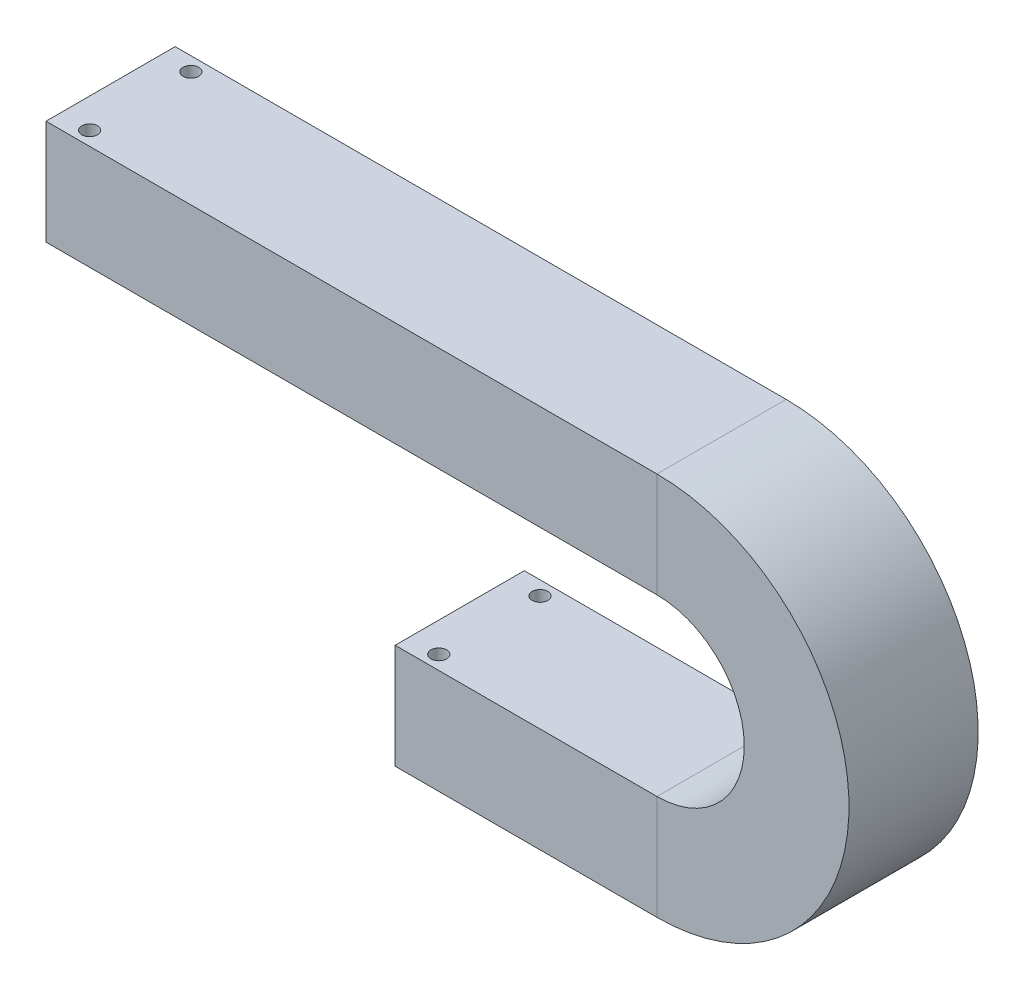
SolidWorks part; units mm, degrees
material "6061-T6"
ref_plane "Front Plane" through (0, 0, 0) normal (0, 0, 1) x (1, 0, 0)
ref_plane "Top Plane" through (0, 0, 0) normal (0, 1, 0) x (1, 0, 0)
ref_plane "Right Plane" through (0, 0, 0) normal (1, 0, 0) x (0, 0, -1)
sketch "Sketch1" plane through (0, 0, 0) normal (1, 0, 0) x (0, 0, -1)
  line L1 (-10, -10) -> (10, -10)
  line L2 (-10, -10) -> (-10, 10)
  line L3 (-10, 10) -> (10, 10)
  line L4 (10, -10) -> (10, 10)
  line L5 (-10, -10) -> (10, 10) construction
  line L6 (-10, 10) -> (10, -10) construction
  line L7 (-18.5, -15) -> (18.5, -15)
  line L8 (-18.5, -15) -> (-18.5, 15)
  line L9 (-18.5, 15) -> (18.5, 15)
  line L10 (18.5, -15) -> (18.5, 15)
  line L11 (-18.5, -15) -> (18.5, 15) construction
  line L12 (-18.5, 15) -> (18.5, -15) construction
  point P0 (0, 0)
  point P6 (0, 0)
  dimension "D1" = 20
  dimension "D2" = 20
  dimension "D3" = 30
  dimension "D4" = 37
sketch "Sketch2" plane through (0, 0, 0) normal (0, 0, 1) x (1, 0, 0)
  line L0 (0, 0) -> (75, 0)
  line L1 (75, 80) -> (-100, 80)
  arc A0 (75, 0) -> (75, 80) centre (75, 40) ccw
  dimension "D1" = 80
  dimension "D2" = 75
  dimension "D3" = 175
sweep "Sweep1" add profiles "Sketch1" path "Sketch2"
hole_wizard "M4 Clearance Hole1" positions "Sketch3" profile "Sketch4" hole size "M4" standard "GB"
sketch "Sketch3" plane through (0, 15, 0) normal (0, 1, 0) x (1, 0, 0)
  line L0 (0, 0) -> (130, 0) construction
  line L1 (130, -18.5) -> (130, 18.5) construction
  line L3 (0, 18.5) -> (0, -18.5) construction
  point P0 (8.5, 14.5)
  point P2 (8.5, -14.5)
  dimension "D1" = 29
  dimension "D2" = 8.5
sketch "Sketch4" plane through (8.5, 15, -14.5) normal (1, 0, 0) x (0, 0, 1)
  line L0 (0, 0) -> (0, 30)
  line L1 (0, 30) -> (2.25, 30)
  line L2 (2.25, 30) -> (2.25, 0)
  line L5 (2.25, 0) -> (0, 0)
  line L11 (0, -6.35) -> (0, 107.95) construction
  dimension "通孔孔直径" = 4.5
  dimension "通孔孔深度" = 30
hole_wizard "M4 Clearance Hole2" positions "Sketch5" profile "Sketch6" hole size "M4" standard "GB" end condition through all
sketch "Sketch5" plane through (0, 95, 0) normal (0, 1, 0) x (1, 0, 0)
  line L0 (-100, 0) -> (130, 0) construction
  line L1 (-100, -18.5) -> (-100, 18.5) construction
  line L2 (130, -18.5) -> (130, 18.5) construction
  point P8 (-91.5, 14.5)
  point P10 (-91.5, -14.5)
  dimension "D1" = 29
  dimension "D2" = 8.5
sketch "Sketch6" plane through (-91.5, 95, 14.5) normal (1, 0, 0) x (0, 0, 1)
  line L0 (0, 0) -> (0, 110)
  line L1 (0, 110) -> (2.25, 110)
  line L2 (2.25, 110) -> (2.25, 0)
  line L5 (2.25, 0) -> (0, 0)
  line L11 (0, -6.35) -> (0, 107.95) construction
  dimension "通孔孔直径" = 4.5
  dimension "通孔孔深度" = 110
